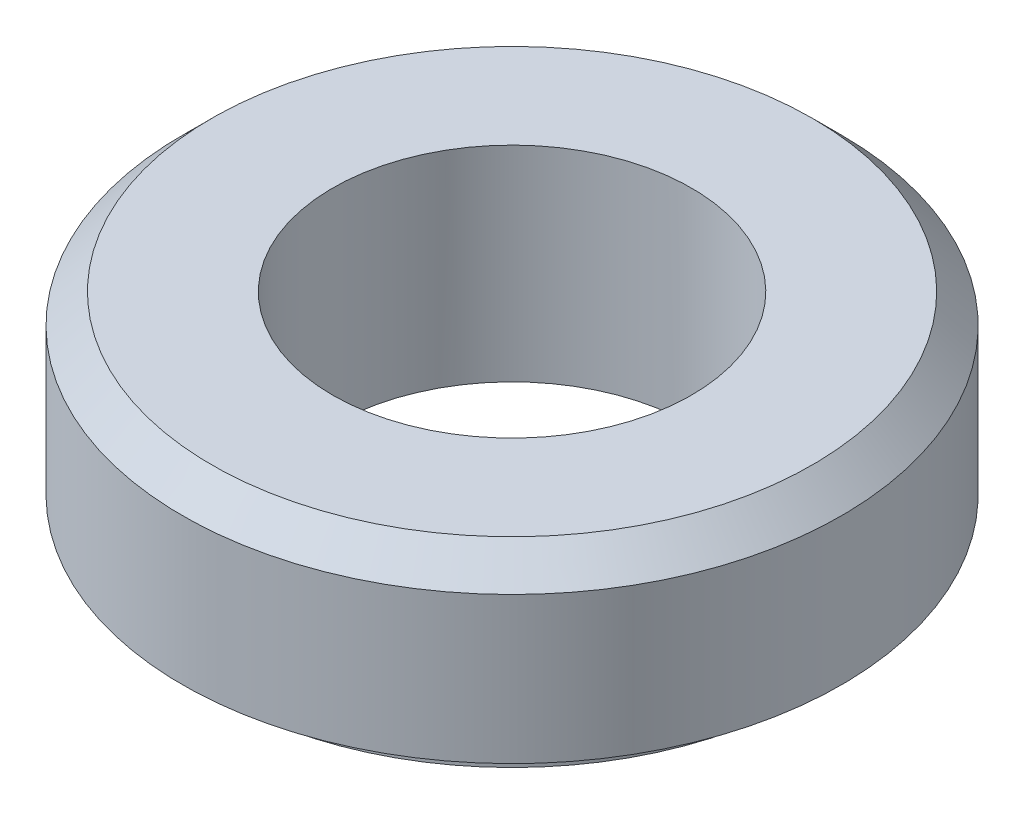
from build123d import *

# Parameters (mm, degrees)
G3_4_TAPPED_HOLE1_D     = 24.5
G3_4_TAPPED_HOLE1_DEPTH = 58.32
G3_4_TAPPED_HOLE1_TIP   = 7.360542583


with BuildPart() as part:
    # Sketch1 → Revolve1 (revolve)
    with BuildSketch(Plane(origin=(0, 0, 0), x_dir=(0, 0, -1), z_dir=(1, 0, 0))):
        Polygon((20, 0), (20, 2), (22.5, 2), (22.5, 12), (20.5, 14), (12, 14), (12, 0), align=None)
    revolve(axis=Axis((0, 0, 0), (0, 1, 0)))

    # G3/4 Tapped Hole1
    with Locations(Plane(origin=(0, 14, 0), x_dir=(1, 0, 0), z_dir=(0, 1, 0))):
        with Locations((0, 0)):
            Hole(G3_4_TAPPED_HOLE1_D / 2, depth=G3_4_TAPPED_HOLE1_DEPTH)
            with Locations((0, 0, -(G3_4_TAPPED_HOLE1_DEPTH + G3_4_TAPPED_HOLE1_TIP / 2))):  # 118° drill point
                Cone(0, G3_4_TAPPED_HOLE1_D / 2, G3_4_TAPPED_HOLE1_TIP, mode=Mode.SUBTRACT)


solid = part.part
